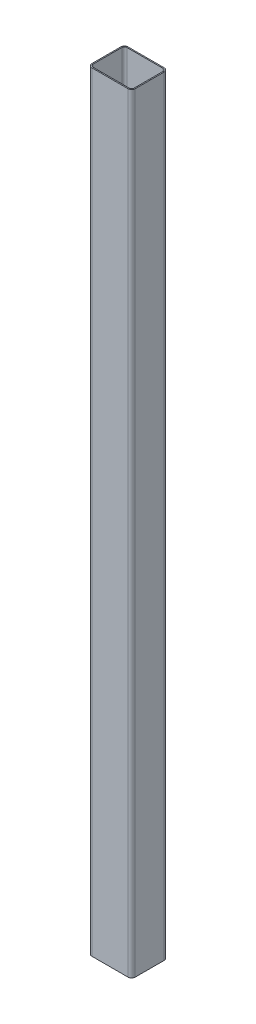
SolidWorks part; units mm, degrees
ref_plane "Front Plane" through (0, 0, 0) normal (0, 0, 1) x (1, 0, 0)
ref_plane "Top Plane" through (0, 0, 0) normal (0, 1, 0) x (1, 0, 0)
ref_plane "Right Plane" through (0, 0, 0) normal (1, 0, 0) x (0, 0, -1)
other "Configuration Table"
sketch "Sketch1" plane through (0, 0, 0) normal (0, 1, 0) x (1, 0, 0)
  line L1 (-50, 50) -> (50, 50)
  line L2 (-60, 40) -> (-60, -40)
  line L3 (-50, -50) -> (50, -50)
  line L4 (60, 40) -> (60, -40)
  line L5 (-60, 50) -> (60, -50) construction
  line L6 (-60, -50) -> (60, 50) construction
  arc A0 (50, 50) -> (60, 40) centre (50, 40) cw
  arc A1 (50, -50) -> (60, -40) centre (50, -40) ccw
  arc A2 (-60, -40) -> (-50, -50) centre (-50, -40) ccw
  arc A3 (-50, 50) -> (-60, 40) centre (-50, 40) ccw
  point P0 (0, 0)
  dimension "D3" = 10
  dimension "D1" = 120
  dimension "D2" = 100
extrude "Extrude-Thin1" add sketch "Sketch1" along normal mid plane 2124 thin
